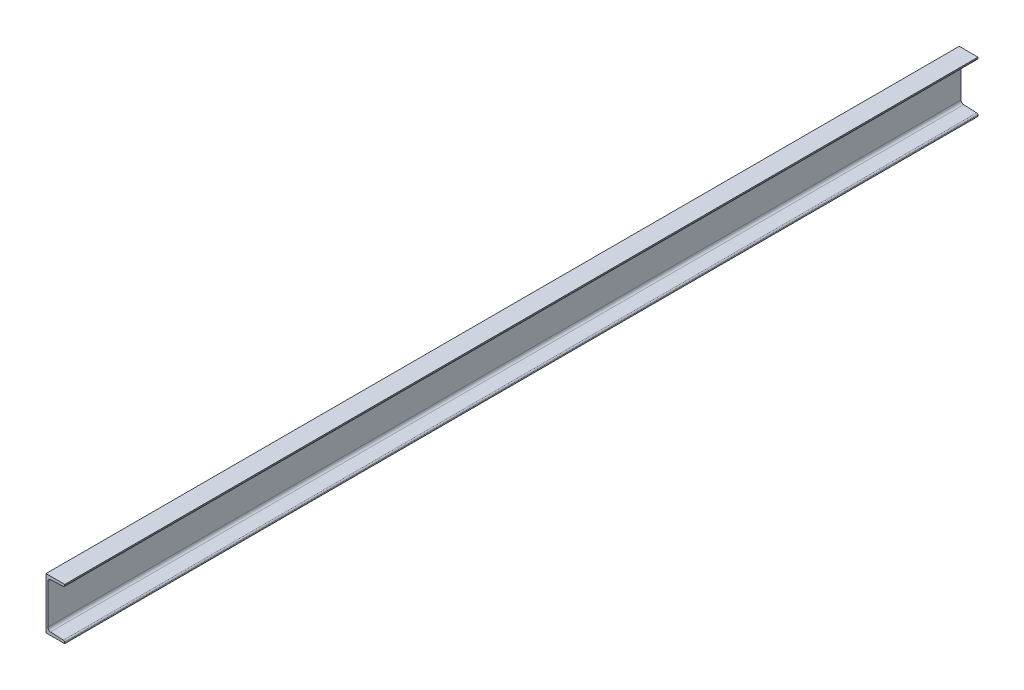
SolidWorks part; units mm, degrees
material "普通碳钢"
ref_plane "Front Plane" through (0, 0, 0) normal (0, 0, 1) x (1, 0, 0)
ref_plane "Top Plane" through (0, 0, 0) normal (0, 1, 0) x (1, 0, 0)
ref_plane "Right Plane" through (0, 0, 0) normal (1, 0, 0) x (0, 0, -1)
sketch "Sketch1" plane through (28.2113, 0, 0) normal (0, 0, 1) x (-1, 0, 0)
  line L0 (28.2113, 0) -> (28.2113, -200)
  line L1 (28.2113, -200) -> (-44.7887, -200)
  line L2 (28.2113, -100) -> (21.2113, -100) construction
  line L3 (21.2113, -177.0757) -> (21.2113, -22.9243)
  line L4 (10.7523, -188.0624) -> (-39.5592, -190.5398)
  line L5 (-44.7887, -196.0332) -> (-44.7887, -200)
  line L6 (21.2113, -187.5473) -> (21.2113, -190.7973) construction
  line L7 (21.2113, -190.7973) -> (-44.7887, -190.7973) construction
  line L8 (-8.2887, -200) -> (-8.2887, -189) construction
  line L9 (-44.7887, -3.9668) -> (-44.7887, 0)
  line L10 (28.2113, 0) -> (-44.7887, 0)
  line L11 (10.7523, -11.9376) -> (-39.5592, -9.4602)
  arc A0 (21.2113, -177.0757) -> (10.7523, -188.0624) centre (10.2113, -177.0757) cw
  arc A1 (10.7523, -11.9376) -> (21.2113, -22.9243) centre (10.2113, -22.9243) cw
  arc A2 (-39.5592, -190.5398) -> (-44.7887, -196.0332) centre (-39.2887, -196.0332) ccw
  arc A3 (-44.7887, -3.9668) -> (-39.5592, -9.4602) centre (-39.2887, -3.9668) ccw
  point P2 (-8.2887, 0)
  point P20 (21.2113, -12.4527)
  point P26 (-44.7887, -9.2027)
  dimension "r" = 11
  dimension "r1" = 5.5
  dimension "h" = 200
  dimension "b" = 73
  dimension "d" = 7
  dimension "t" = 11
  dimension "D5" = 66
  dimension "D6" = 3.25
extrude "Boss-Extrude1" add sketch "Sketch1" along normal mid plane 3556
